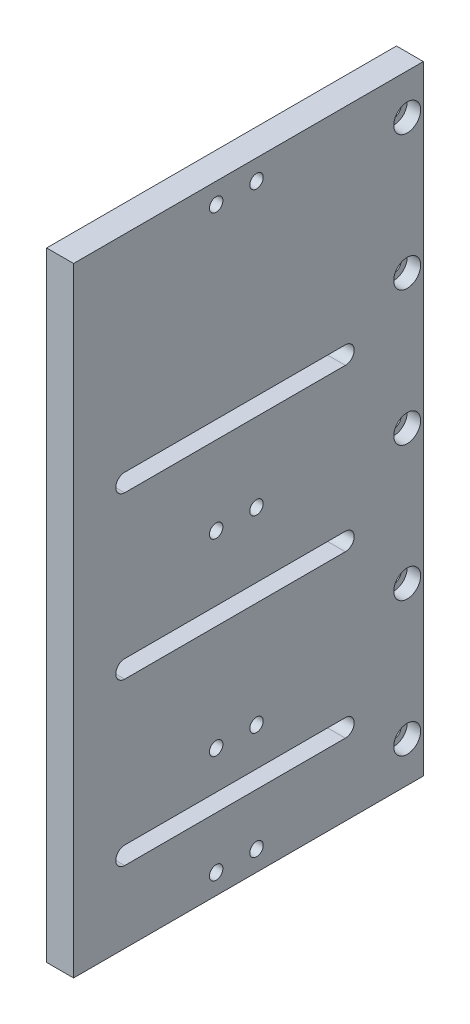
SolidWorks part; units mm, degrees
ref_plane "Front Plane" through (0, 0, 0) normal (0, 0, 1) x (1, 0, 0)
ref_plane "Top Plane" through (0, 0, 0) normal (0, 1, 0) x (1, 0, 0)
ref_plane "Right Plane" through (0, 0, 0) normal (1, 0, 0) x (0, 0, -1)
sketch "Sketch 1" plane through (0, 0, 0) normal (1, 0, 0) x (0, 0, -1)
  line L1 (-65, -115) -> (65, -115)
  line L2 (-65, -115) -> (-65, 115)
  line L3 (-65, 115) -> (65, 115)
  line L4 (65, -115) -> (65, 115)
  line L5 (-65, -115) -> (65, 115) construction
  line L6 (-65, 115) -> (65, -115) construction
  point P0 (0, 0)
  dimension "D1" = 130
  dimension "D2" = 230
extrude "Boss-Extrude 1" add sketch "Sketch 1" along normal blind 10
hole_wizard "M6 Tapped Hole 1" positions "Sketch 3" profile "Sketch 2" tap size "M6" standard "GB" end condition through all
sketch "Sketch 3" plane through (0, 0, 0) normal (-1, 0, 0) x (0, 0, 1)
  line L0 (65, 115) -> (65, -115) construction
  line L1 (65, -115) -> (-65, -115) construction
  point P0 (12, -107.5)
  dimension "D1" = 53
  dimension "D2" = 7.5
sketch "Sketch 2" plane through (0, -107.5, 12) normal (0, 1, 0) x (0, 0, 1)
  line L0 (0, 0) -> (0, 10)
  line L1 (0, 10) -> (2.5, 10)
  line L2 (2.5, 10) -> (2.5, 0)
  line L5 (2.5, 0) -> (0, 0)
  line L11 (0, -6.35) -> (0, 107.95) construction
  dimension "貫穿螺孔鑽直徑" = 5
  dimension "貫穿螺孔鑽深度" = 10
cosmetic thread "Cosmetic Thread 1" parameters "D2"=6
pattern_linear "Linear Pattern 1" count 2 spacing 15 along (0, 0, -1) of "M6 Tapped Hole 1"
hole_wizard "M5 Socket Head Cap Screw Counterbore 1" positions "Sketch 5" profile "Sketch 4" counterbore size "M5" standard "JIS" end condition through all
sketch "Sketch 5" plane through (10, 0, 0) normal (1, 0, 0) x (0, 0, -1)
  line L0 (65, -115) -> (65, 115) construction
  point P0 (59, 0)
  point P4 (65, 0)
  dimension "D1" = 6
  dimension "D2" = 0
sketch "Sketch 4" plane through (10, 0, -59) normal (0, 1, 0) x (0, 0, -1)
  line L0 (0, 0) -> (0, 10)
  line L1 (0, 10) -> (2.75, 10)
  line L3 (2.75, 10) -> (2.75, 5)
  line L4 (2.75, 5) -> (5, 5)
  line L5 (5, 5) -> (5, 0)
  line L7 (5, 0) -> (0, 0)
  line L11 (0, -6.35) -> (0, 107.95) construction
  dimension "貫穿孔直徑" = 5.5
  dimension "貫穿孔深度" = 10
  dimension "柱孔直徑" = 10
  dimension "柱孔深度" = 5
pattern_linear "Linear Pattern 2" count 3 spacing 50 along (0, 1, 0) count 3 spacing 50 along (0, -1, 0) seed only of "M5 Socket Head Cap Screw Counterbore 1"
pattern_linear "Linear Pattern 3" count 2 spacing 110 along (0, 1, 0) of "Linear Pattern 1", "M6 Tapped Hole 1"
pattern_linear "Linear Pattern 4" count 2 spacing 215 along (0, 1, 0) of "Linear Pattern 1", "M6 Tapped Hole 1"
sketch "Sketch 8" plane through (0, 0, 0) normal (-1, 0, 0) x (0, 0, 1)
  line L0 (-36, -85) -> (46, -85) construction
  line L1 (-36, -81.7) -> (46, -81.7)
  line L2 (-36, -88.3) -> (46, -88.3)
  line L3 (65, -115) -> (-65, -115) construction
  line L4 (-65, -115) -> (-65, 115) construction
  arc A0 (-36, -81.7) -> (-36, -88.3) centre (-36, -85) ccw
  arc A1 (46, -88.3) -> (46, -81.7) centre (46, -85) ccw
  point P2 (5, -85)
  dimension "D1" = 6.6
  dimension "D2" = 82
  dimension "D3" = 30
  dimension "D4" = 29
extrude "Cut-Extrude 1" cut sketch "Sketch 8" against normal through all
pattern_linear "Linear Pattern 8" count 3 spacing 60 along (0, 1, 0) of "Cut-Extrude 1"
pattern_linear "Linear Pattern 7" count 2 spacing 40 along (0, 1, 0) of "Linear Pattern 1", "M6 Tapped Hole 1"
